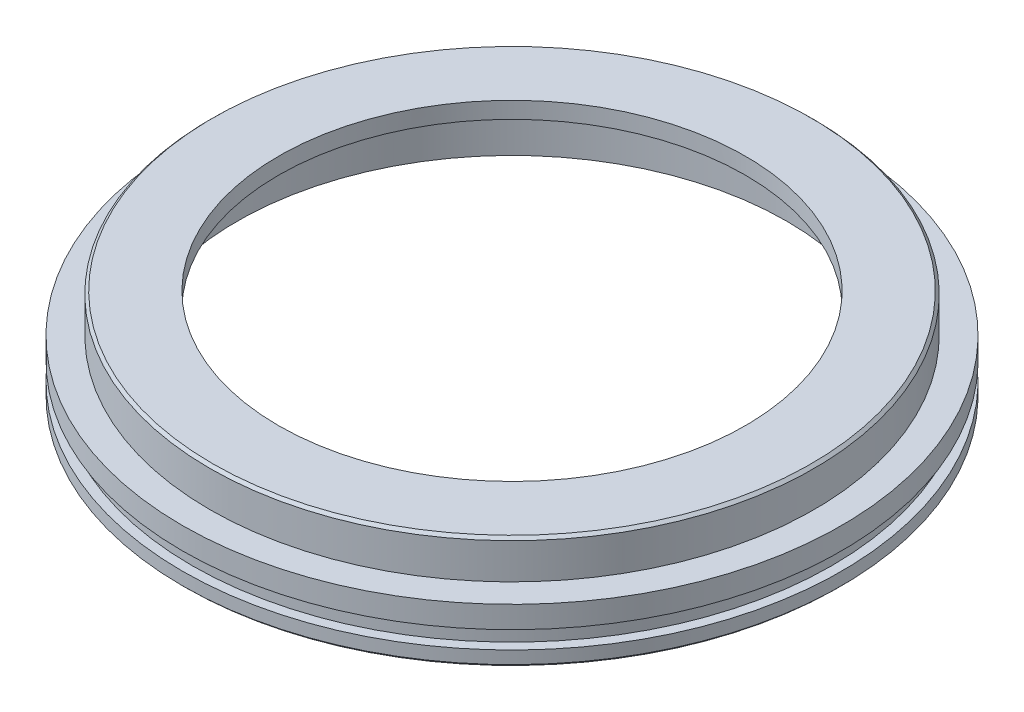
SolidWorks part; units mm, degrees
material "普通碳钢"
ref_plane "Front Plane" through (0, 0, 0) normal (0, 0, 1) x (1, 0, 0)
ref_plane "Top Plane" through (0, 0, 0) normal (0, 1, 0) x (1, 0, 0)
ref_plane "Right Plane" through (0, 0, 0) normal (1, 0, 0) x (0, 0, -1)
sketch "Sketch1" plane through (0, 0, 0) normal (0, 1, 0) x (1, 0, 0)
  circle A0 centre (0, 0) radius 60
  dimension "D1" = 120
extrude "Boss-Extrude1" add sketch "Sketch1" along normal blind 10
sketch "Sketch2" plane through (0, 10, 0) normal (0, 1, 0) x (1, 0, 0)
  circle A0 centre (0, 0) radius 55
  dimension "D1" = 110
extrude "Boss-Extrude2" add sketch "Sketch2" along normal blind 7
sketch "Sketch3" plane through (0, 17, 0) normal (0, 1, 0) x (1, 0, 0)
  circle A0 centre (0, 0) radius 42.5
  dimension "D1" = 85
extrude "Cut-Extrude1" cut sketch "Sketch3" against normal through all
sketch "Sketch4" plane through (0, 0, 0) normal (0, -1, 0) x (1, 0, 0)
  circle A0 centre (0, 0) radius 55
  dimension "D1" = 110
extrude "Cut-Extrude2" cut sketch "Sketch4" against normal blind 3
sketch "Sketch5" plane through (0, 3, 0) normal (0, -1, 0) x (1, 0, 0)
  circle A0 centre (0, 0) radius 50
  dimension "D1" = 100
extrude "Cut-Extrude3" cut sketch "Sketch5" against normal blind 11
ref_plane "Plane1" through (0, 6, 0) normal (0, -1, 0) x (-1, 0, 0)
sketch "Sketch6" plane through (0, 6, 0) normal (0, -1, 0) x (-1, 0, 0)
  circle A0 centre (0, 0) radius 58.25
  dimension "D1" = 116.5
extrude "Cut-Extrude4" cut sketch "Sketch6" along normal blind 3.2 flip side to cut
chamfer "Chamfer1" distance 0.5 angle 45 1 edges at (0, 0, 60)
chamfer "Chamfer2" distance 0.5 angle 45 1 edges at (0, 17, 55)
